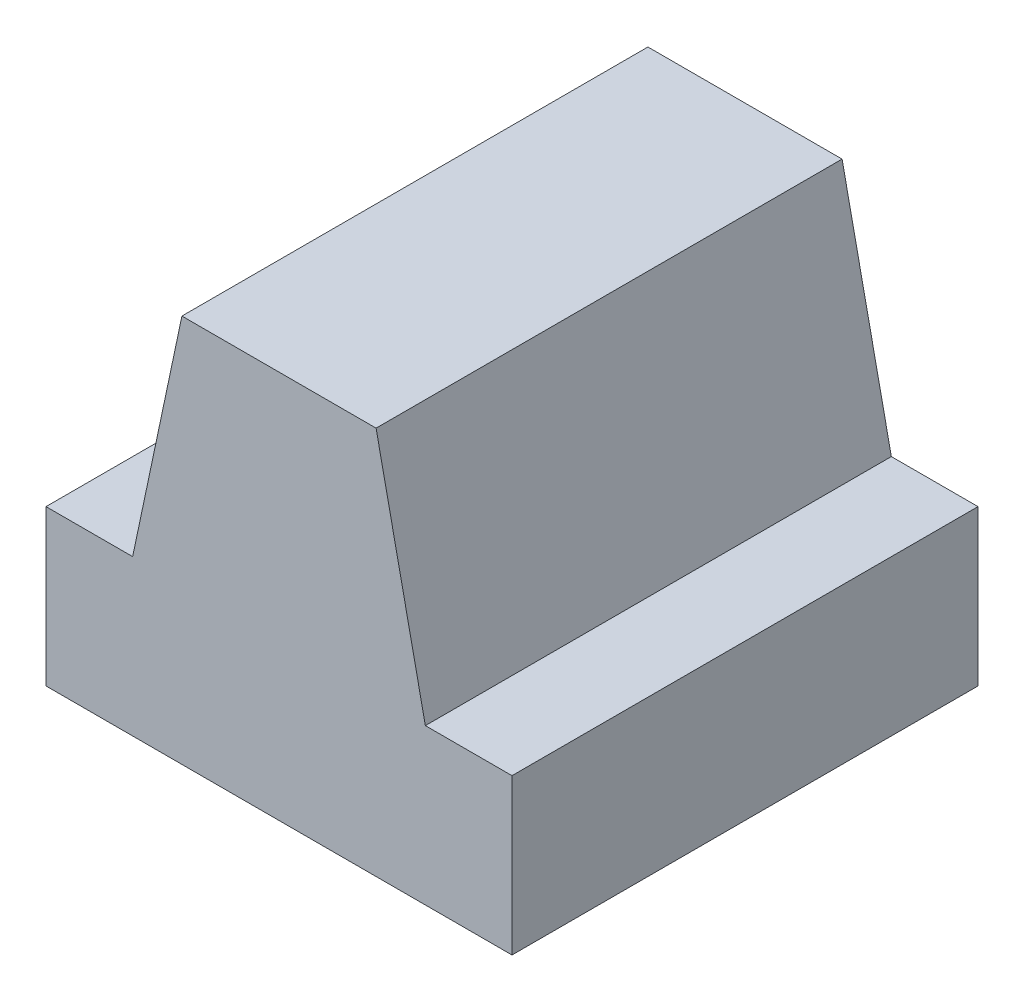
SolidWorks part; units mm, degrees
ref_plane "Front Plane" through (0, 0, 0) normal (0, 0, 1) x (1, 0, 0)
ref_plane "Top Plane" through (0, 0, 0) normal (0, 1, 0) x (1, 0, 0)
ref_plane "Right Plane" through (0, 0, 0) normal (1, 0, 0) x (0, 0, -1)
other "Configuration Table"
sketch "Sketch1" plane through (0, 0, 0) normal (0, 0, 1) x (1, 0, 0)
  line L0 (0, 0) -> (0, 14027.3196) construction
  line L1 (-1.25, 5) -> (1.25, 5)
  line L3 (3, 2) -> (3, 0)
  line L4 (3, 0) -> (-3, 0)
  line L5 (-3, 0) -> (-3, 2)
  line L7 (-3, 2) -> (-1.8844, 2)
  line L8 (-1.8844, 2) -> (-1.25, 5)
  line L9 (-1.25, 5) -> (1.25, 5)
  line L10 (1.25, 5) -> (1.8844, 2)
  line L11 (1.8844, 2) -> (3, 2)
  dimension "D1" = 6
  dimension "D2" = 2
  dimension "D3" = 5
  dimension "D4" = 2.5
extrude "Boss-Extrude1" add sketch "Sketch1" along normal blind 6 contours L4 L0 L1 L8 L7 L5 | L0 L4 L3 L11 L10 L9
sketch "Sketch3" plane through (0, 0, 0) normal (0, -1, 0) x (1, 0, 0)
  line L0 (-3, 3) -> (3, 3)
  line L3 (-3, 6) -> (-3, 0) construction
  line L4 (3, 6) -> (3, 0) construction
